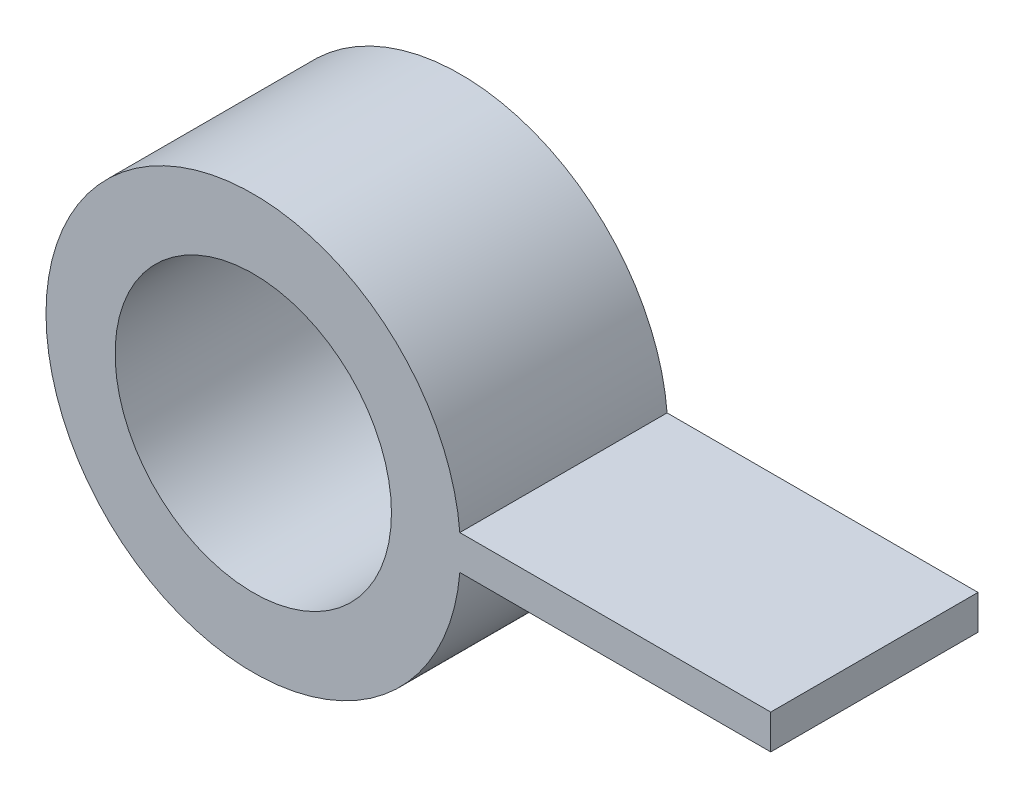
from build123d import *

# Parameters (mm, degrees)
SKETCH_1_R      = 12
SKETCH_1_R_2    = 8
EXTRUDE_1_DEPTH = 6
SKETCH_2_W      = 18
SKETCH_2_H      = 2
EXTRUDE_2_DEPTH = 12


with BuildPart() as part:
    # 草图1 → 凸台-拉伸1 (new, symmetric)
    with BuildSketch(Plane.XY):
        Circle(SKETCH_1_R)
        Circle(SKETCH_1_R_2, mode=Mode.SUBTRACT)
    extrude(amount=EXTRUDE_1_DEPTH, both=True)

    # 草图2 → 凸台-拉伸2 (add)
    with BuildSketch(Plane.XY.offset(6)):
        with Locations((20.958260743, 0)):
            Rectangle(SKETCH_2_W, SKETCH_2_H)
    extrude(amount=-EXTRUDE_2_DEPTH)


solid = part.part
